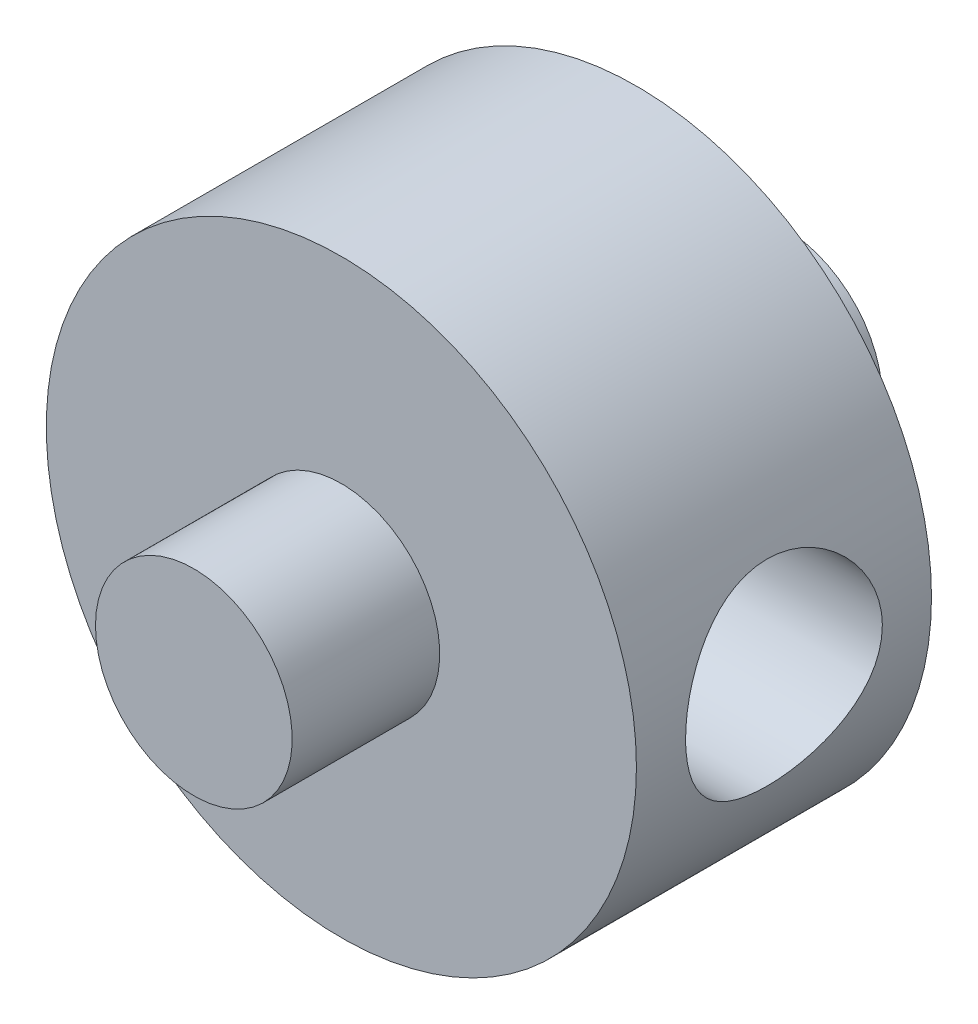
SolidWorks part; units mm, degrees
ref_plane "Front Plane" through (0, 0, 0) normal (0, 0, 1) x (1, 0, 0)
ref_plane "Top Plane" through (0, 0, 0) normal (0, 1, 0) x (1, 0, 0)
ref_plane "Right Plane" through (0, 0, 0) normal (1, 0, 0) x (0, 0, -1)
sketch "Sketch1" plane through (0, 0, 0) normal (0, 0, 1) x (1, 0, 0)
  circle A0 centre (0, 0) radius 9.525
  dimension "D1" = 19.05
extrude "Boss-Extrude1" add sketch "Sketch1" against normal blind 9.525
sketch "Sketch2" plane through (0, 0, 0) normal (0, 0, 1) x (1, 0, 0)
  circle A0 centre (0, 0) radius 3.175
  dimension "D1" = 6.35
extrude "Boss-Extrude2" add sketch "Sketch2" along normal blind 4.7625
sketch "Sketch3" plane through (0, 0, -9.525) normal (0, 0, -1) x (-1, 0, 0)
  circle A0 centre (0, 0) radius 3.175
  dimension "D1" = 6.35
extrude "Boss-Extrude3" add sketch "Sketch3" along normal blind 4.7625
sketch "Sketch4" plane through (0, 0, 0) normal (1, 0, 0) x (0, 0, -1)
  line L0 (9.525, -3.175) -> (9.525, 3.175) construction
  circle A0 centre (4.7625, 0) radius 3.175
  dimension "D1" = 6.35
  dimension "D2" = 4.7625
extrude "Cut-Extrude1" cut sketch "Sketch4" along normal through all
